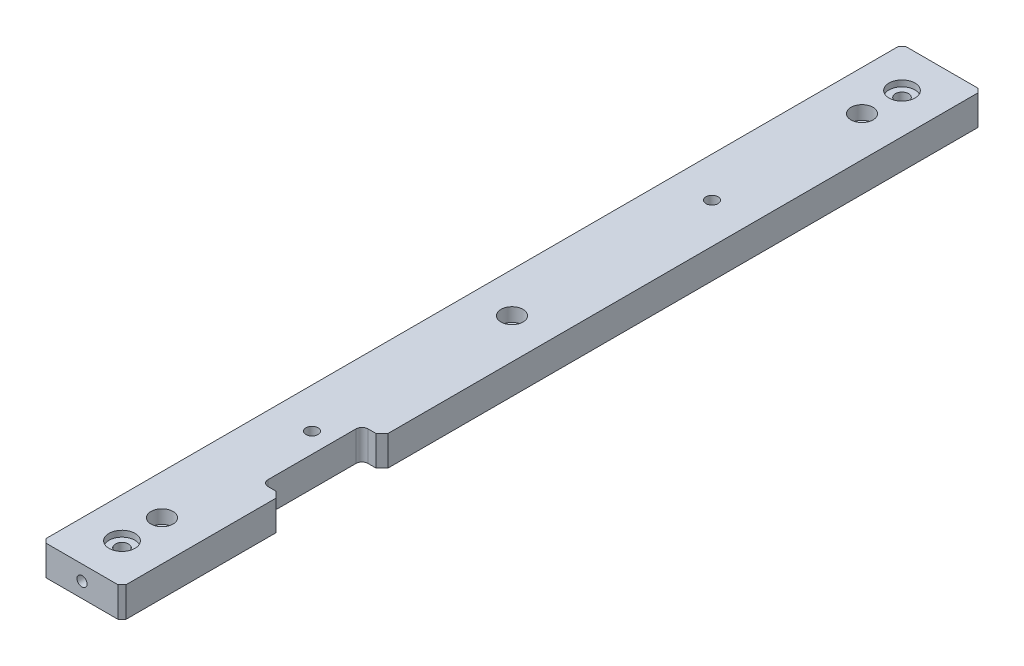
SolidWorks part; units mm, degrees
material "A5052"
ref_plane "Front Plane" through (0, 0, 0) normal (0, 0, 1) x (1, 0, 0)
ref_plane "Top Plane" through (0, 0, 0) normal (0, 1, 0) x (1, 0, 0)
ref_plane "Right Plane" through (0, 0, 0) normal (1, 0, 0) x (0, 0, -1)
sketch "Sketch1" plane through (0, 0, 0) normal (0, 1, 0) x (1, 0, 0)
  line L1 (20, 215) -> (-20, 215)
  line L2 (20, 215) -> (20, -215)
  line L3 (20, -215) -> (-20, -215)
  line L4 (-20, 215) -> (-20, -215)
  line L5 (20, 215) -> (-20, -215) construction
  line L6 (20, -215) -> (-20, 215) construction
  point P0 (0, 0)
  dimension "D1" = 40
  dimension "D2" = 430
extrude "Boss-Extrude1" add sketch "Sketch1" along normal mid plane 15
sketch "Sketch2" plane through (0, 7.5, 0) normal (0, 1, 0) x (1, 0, 0)
  line L0 (0, 0) -> (0, 195) construction
  line L1 (20, 215) -> (-20, 215) construction
  line L2 (0, 0) -> (43.891, 0) construction
  circle A0 centre (0, 195) radius 6.5
  circle A1 centre (0, -195) radius 6.5
  dimension "D1" = 13
  dimension "D2" = 20
extrude "Cut-Extrude1" cut sketch "Sketch2" against normal blind 3
hole_wizard "Hex socket cap screw hole type 1" positions "Sketch3" profile "Sketch4" counterbore size "M6" standard "GB" end condition through all
sketch "Sketch3" plane through (0, -7.5, 0) normal (0, -1, 0) x (-1, 0, 0)
  point P0 (0, -195)
  point P3 (0, 195)
sketch "Sketch4" plane through (0, -7.5, 195) normal (1, 0, 0) x (0, 0, -1)
  line L0 (0, 0) -> (0, 15)
  line L1 (0, 15) -> (3.3, 15)
  line L3 (3.3, 15) -> (3.3, 6.8)
  line L4 (3.3, 6.8) -> (5.5, 6.8)
  line L5 (5.5, 6.8) -> (5.5, 0)
  line L7 (5.5, 0) -> (0, 0)
  line L11 (0, -6.35) -> (0, 107.95) construction
  dimension "通孔孔直径" = 6.6
  dimension "通孔孔深度" = 15
  dimension "柱形沉头孔直径" = 11
  dimension "柱形沉头孔深度" = 6.8
hole_wizard "M5 Tapped Hole1" positions "Sketch5" profile "Sketch6" tap size "M5" standard "GB"
sketch "Sketch5" plane through (-20, 0, 0) normal (-1, 0, 0) x (0, 0, 1)
  line L1 (0, 0) -> (-195, 0) construction
  line L4 (0, 0) -> (0, 27.881) construction
  point P0 (-195, 0)
  point P21 (195, 0)
  point P23 (-65, 0)
  point P25 (65, 0)
  dimension "D1" = 130
  dimension "D2" = 130
sketch "Sketch6" plane through (-20, 0, -195) normal (0, 1, 0) x (0, 0, 1)
  line L0 (0, 0) -> (0, 16.2618)
  line L1 (0, 16.2618) -> (2.1, 15)
  line L2 (2.1, 15) -> (2.1, 0)
  line L5 (2.1, 0) -> (0, 0)
  line L10 (0, 16.2618) -> (-2.1, 15) construction
  line L11 (0, -6.35) -> (0, 107.95) construction
  dimension "螺纹孔钻头直径" = 4.2
  dimension "螺纹孔钻头深度" = 15
  dimension "导头角度" = 118
cosmetic thread "Hole thread 1" parameters "D1"=10, "D2"=5
cosmetic thread "Hole thread 2" parameters "D1"=10, "D2"=5
cosmetic thread "Hole thread 3" parameters "D1"=10, "D2"=5
cosmetic thread "Hole thread 6" parameters "D1"=10, "D2"=5
chamfer "Chamfer1" distance 2 angle 45 4 edges at (20, 0, -215) (-20, 0, -215) (20, 0, 215) (-20, 0, 215)
hole_wizard "Hex socket cap screw hole type 2" positions "Sketch7" profile "Sketch8" counterbore size "M6" standard "GB" end condition through all
sketch "Sketch7" plane through (0, 7.5, 0) normal (0, 1, 0) x (1, 0, 0)
  line L0 (0, 0) -> (20, 0) construction
  line L1 (20, -213) -> (20, 213) construction
  line L4 (0, 0) -> (0, 175) construction
  point P0 (0, 175)
  point P20 (0, -175)
  point P23 (0, 0)
  dimension "D1" = 350
sketch "Sketch8" plane through (0, 7.5, -175) normal (1, 0, 0) x (0, 0, 1)
  line L0 (0, 0) -> (0, 15)
  line L1 (0, 15) -> (3.3, 15)
  line L3 (3.3, 15) -> (3.3, 6.8)
  line L4 (3.3, 6.8) -> (5.5, 6.8)
  line L5 (5.5, 6.8) -> (5.5, 0)
  line L7 (5.5, 0) -> (0, 0)
  line L11 (0, -6.35) -> (0, 107.95) construction
  dimension "通孔孔直径" = 6.6
  dimension "通孔孔深度" = 15
  dimension "柱形沉头孔直径" = 11
  dimension "柱形沉头孔深度" = 6.8
hole_wizard "M6 Tapped Hole1" positions "Sketch9" profile "Sketch10" tap size "M6" standard "GB"
sketch "Sketch9" plane through (0, 0, 215) normal (0, 0, 1) x (1, 0, 0)
  point P0 (0, 0)
sketch "Sketch10" plane through (0, 0, 215) normal (1, 0, 0) x (0, -1, 0)
  line L0 (0, 0) -> (0, 14.5022)
  line L1 (0, 14.5022) -> (2.5, 13)
  line L2 (2.5, 13) -> (2.5, 0)
  line L5 (2.5, 0) -> (0, 0)
  line L10 (0, 14.5022) -> (-2.5, 13) construction
  line L11 (0, -6.35) -> (0, 107.95) construction
  dimension "螺纹孔钻头直径" = 5
  dimension "螺纹孔钻头深度" = 13
  dimension "导头角度" = 118
cosmetic thread "Hole thread 4" parameters "D1"=10, "D2"=6
hole_wizard "M6 Tapped Hole2" positions "Sketch11" profile "Sketch12" tap size "M6" standard "GB"
sketch "Sketch11" plane through (0, 0, -215) normal (0, 0, -1) x (-1, 0, 0)
  point P0 (0, 0)
sketch "Sketch12" plane through (0, 0, -215) normal (1, 0, 0) x (0, 1, 0)
  line L0 (0, 0) -> (0, 14.5022)
  line L1 (0, 14.5022) -> (2.5, 13)
  line L2 (2.5, 13) -> (2.5, 0)
  line L5 (2.5, 0) -> (0, 0)
  line L10 (0, 14.5022) -> (-2.5, 13) construction
  line L11 (0, -6.35) -> (0, 107.95) construction
  dimension "螺纹孔钻头直径" = 5
  dimension "螺纹孔钻头深度" = 13
  dimension "导头角度" = 118
cosmetic thread "Hole thread 5" parameters "D1"=10, "D2"=6
hole_wizard "Ø6.0 (6) Diameter Hole1" positions "Sketch13" profile "Sketch14" hole size "Ø6.0" standard "GB"
sketch "Sketch13" plane through (0, -7.5, 0) normal (0, -1, 0) x (-1, 0, 0)
  line L0 (0, 0) -> (17.764, 0) construction
  point P0 (0, 100)
  point P2 (0, -100)
  dimension "D1" = 200
sketch "Sketch14" plane through (0, -7.5, -100) normal (1, 0, 0) x (0, 0, -1)
  line L0 (0, 0) -> (0, 18.8026)
  line L1 (0, 18.8026) -> (3, 17)
  line L2 (3, 17) -> (3, 0)
  line L5 (3, 0) -> (0, 0)
  line L10 (0, 18.8026) -> (-3, 17) construction
  line L11 (0, -6.35) -> (0, 107.95) construction
  dimension "孔直径" = 6
  dimension "孔深度" = 17
  dimension "导头角度" = 118
sketch "Sketch15" plane through (0, -7.5, 0) normal (0, -1, 0) x (1, 0, 0)
  line L0 (20, 213) -> (20, -213) construction
  line L1 (20, 85) -> (10, 85)
  line L2 (20, 85) -> (20, 135)
  line L3 (20, 135) -> (10, 135)
  line L4 (10, 85) -> (10, 135)
  line L5 (-18, 215) -> (18, 215) construction
  dimension "D1" = 10
  dimension "D2" = 80
  dimension "D3" = 50
extrude "Cut-Extrude2" cut sketch "Sketch15" against normal through all
fillet "Fillet1" radius 3 2 edges at (10, 0, 135) (10, 0, 85)
chamfer "Chamfer2" distance 3 angle 45 2 edges at (20, 0, 135) (20, 0, 85)
